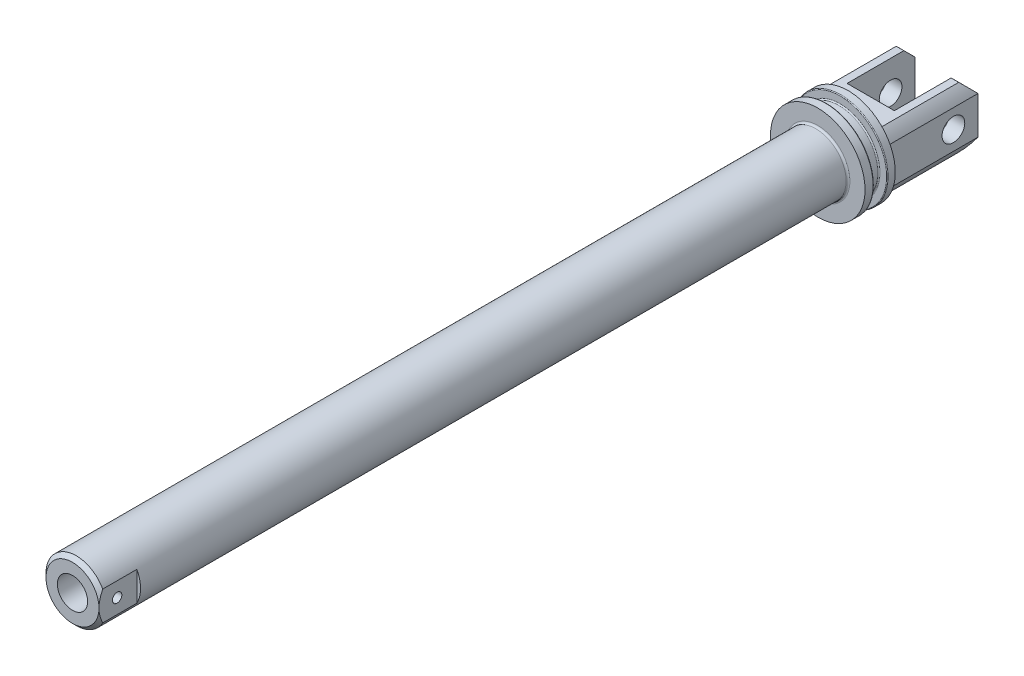
from build123d import *

# Parameters (mm, degrees)
SKETCH1_R               = 8
BOSS_EXTRUDE1_DEPTH     = 197
SKETCH2_R               = 12.5
BOSS_EXTRUDE2_DEPTH     = 8
SKETCH3_W               = 2.25
SKETCH3_H               = 3.6
SKETCH8_R               = 11.5
BOSS_EXTRUDE4_DEPTH     = 24
CUT_EXTRUDE1_DEPTH      = 198.791556948
CUT_EXTRUDE1_DEPTH_BACK = 198.791556948
SKETCH10_W              = 12.5
SKETCH10_H              = 21.605782088
CUT_EXTRUDE3_DEPTH      = 231.593256623
CUT_EXTRUDE3_DEPTH_BACK = 231.593256623
CUT_EXTRUDE5_START      = -24
CUT_EXTRUDE5_DEPTH      = 24
FILLET1_R               = 0.5
FILLET2_R               = 0.2
FILLET3_R               = 0.3
CHAMFER3_SIZE           = 1
CUT_EXTRUDE7_DEPTH      = 199.457804086
CUT_EXTRUDE7_DEPTH_BACK = 199.457804086
SKETCH15_W              = 2.199256875
SKETCH15_H              = 8
SKETCH15_W_2            = 2.880068719
SKETCH15_H_2            = 10
SKETCH14_R              = 3
CUT_EXTRUDE6_DEPTH      = 24
HOLE2_D                 = 8
HOLE2_DEPTH             = 7.5
M6_TAPPED_HOLE1_D       = 5
M6_TAPPED_HOLE1_DEPTH   = 18
M6_TAPPED_HOLE1_TIP     = 1.502151548
M3_TAPPED_HOLE1_D       = 2.5
M3_TAPPED_HOLE1_DEPTH   = 7.5
M3_TAPPED_HOLE1_TIP     = 0.751075774


with BuildPart() as part:
    # Sketch1 → Boss-Extrude1 (new body)
    with BuildSketch(Plane.XY):
        Circle(SKETCH1_R)
    extrude(amount=BOSS_EXTRUDE1_DEPTH)

    # Sketch2 → Boss-Extrude2 (add)
    with BuildSketch(Plane(origin=(0, 0, 0), x_dir=(-1, 0, 0), z_dir=(0, 0, -1))):
        Circle(SKETCH2_R)
    extrude(amount=BOSS_EXTRUDE2_DEPTH)

    # Sketch3 → Cut-Revolve1 (revolve, cut)
    with BuildSketch(Plane(origin=(0, 0, 0), x_dir=(1, 0, 0), z_dir=(0, 1, 0))):
        with Locations((-11.375, 4.1)):
            Rectangle(SKETCH3_W, SKETCH3_H)
    revolve(axis=Axis((0, 0, -10.00817261), (0, 0, 1)), mode=Mode.SUBTRACT)

    # Sketch8 → Boss-Extrude4 (add)
    with BuildSketch(Plane(origin=(0, 0, -8), x_dir=(-1, 0, 0), z_dir=(0, 0, -1))):
        Circle(SKETCH8_R)
    extrude(amount=BOSS_EXTRUDE4_DEPTH)

    # Sketch10 → Cut-Extrude1 (cut, two sides: drawn at the far end of the back side and taken through both)
    with BuildSketch(Plane(origin=(0, 0, 0), x_dir=(1, 0, 0), z_dir=(0, 1, 0)).offset(-CUT_EXTRUDE1_DEPTH_BACK)):
        with Locations((0, 24.802891044)):
            Rectangle(SKETCH10_W, SKETCH10_H)
    extrude(amount=CUT_EXTRUDE1_DEPTH + CUT_EXTRUDE1_DEPTH_BACK, mode=Mode.SUBTRACT)

    # Sketch11 → Cut-Extrude3 (cut, two sides: drawn at the far end of the back side and taken through both)
    with BuildSketch(Plane(origin=(0, -11.5, -32), x_dir=(0, 0, -1), z_dir=(-1, 0, 0)).offset(-CUT_EXTRUDE3_DEPTH_BACK)):
        Polygon((0.010981051, -16.5), (-3, -19.5), (-24, -19.5), (-24, -26.396557876), (1.498378991, -26.396557876), (1.498378991, -19.5), (0.010981051, -19.5), align=None)
        Polygon((-24, -3.5), (-24, 3.359688932), (2.769529036, 3.359688932), (2.769529036, -3.5), (1.498378991, -3.5), (0.010981051, -3.5), (0.010981051, -6.5), (-3, -3.5), align=None)
    extrude(amount=CUT_EXTRUDE3_DEPTH + CUT_EXTRUDE3_DEPTH_BACK, mode=Mode.SUBTRACT)

    # Sketch13 → Cut-Extrude5 (cut)
    with BuildSketch(Plane(origin=(0, 0, -32), x_dir=(-1, 0, 0), z_dir=(0, 0, -1)).offset(CUT_EXTRUDE5_START)):
        with BuildLine():
            Line((10.356157589, -5), (10.356157589, 5))
            ThreePointArc((10.356157589, 5), (11.5, 0), (10.356157589, -5))
        make_face()
        with BuildLine():
            Line((-10.356157589, -5), (-10.356157589, 5))
            ThreePointArc((-10.356157589, 5), (-11.5, 0), (-10.356157589, -5))
        make_face()
    extrude(amount=CUT_EXTRUDE5_DEPTH, mode=Mode.SUBTRACT)

    # Fillet1
    fillet1_edges = [part.edges().sort_by_distance(p)[0] for p in [
        (-8, 0, 0),
    ]]
    fillet(fillet1_edges, radius=FILLET1_R)

    # Fillet2
    fillet2_edges = [part.edges().sort_by_distance(p)[0] for p in [
        (12.5, 0, -2.3),
        (12.5, 0, -5.9),
    ]]
    fillet(fillet2_edges, radius=FILLET2_R)

    # Fillet3
    fillet3_edges = [part.edges().sort_by_distance(p)[0] for p in [
        (10.25, 0, -2.3),
        (10.25, 0, -5.9),
    ]]
    fillet(fillet3_edges, radius=FILLET3_R)

    # Chamfer3
    chamfer3_edges = [part.edges().sort_by_distance(p)[0] for p in [
        (-8, 0, 197),
    ]]
    chamfer(chamfer3_edges, length=CHAMFER3_SIZE)

    # Sketch15 → Cut-Extrude7 (cut, two sides: drawn at the far end of the back side and taken through both)
    with BuildSketch(Plane(origin=(0, 8, 0), x_dir=(1, 0, 0), z_dir=(0, 1, 0)).offset(-CUT_EXTRUDE7_DEPTH_BACK)):
        with Locations((-8.099628438, -191)):
            Rectangle(SKETCH15_W, SKETCH15_H)
        with BuildLine():
            Line((-8.5, -153.05), (-9.470215056, -153.05))
            Line((-9.470215056, -153.05), (-9.470215056, -177.95))
            Line((-9.470215056, -177.95), (-8.5, -177.95))
            ThreePointArc((-8.5, -177.95), (-6.732233047, -177.217766953), (-6, -175.45))
            Line((-6, -175.45), (-6, -155.55))
            ThreePointArc((-6, -155.55), (-6.732233047, -153.782233047), (-8.5, -153.05))
        make_face()
        with Locations((8.44003436, -192)):
            Rectangle(SKETCH15_W_2, SKETCH15_H_2)
    extrude(amount=CUT_EXTRUDE7_DEPTH + CUT_EXTRUDE7_DEPTH_BACK, mode=Mode.SUBTRACT)

    # Sketch14 → Cut-Extrude6 (cut)
    with BuildSketch(Plane(origin=(10.356157589, 0, 0), x_dir=(0, 0, -1), z_dir=(1, 0, 0))):
        with Locations(Location((25.5, 0, 0), (0, 0, 90))):
            Circle(SKETCH14_R)
    extrude(amount=-CUT_EXTRUDE6_DEPTH, mode=Mode.SUBTRACT)

    # Hole2
    with Locations(Plane.XY.offset(197)):
        with Locations((0, 0)):
            Hole(HOLE2_D / 2, depth=HOLE2_DEPTH)

    # M6 Tapped Hole1
    with Locations(Plane.XY.offset(197)):
        with Locations((0, 0)):
            Hole(M6_TAPPED_HOLE1_D / 2, depth=M6_TAPPED_HOLE1_DEPTH)
            with Locations((0, 0, -(M6_TAPPED_HOLE1_DEPTH + M6_TAPPED_HOLE1_TIP / 2))):  # 118° drill point
                Cone(0, M6_TAPPED_HOLE1_D / 2, M6_TAPPED_HOLE1_TIP, mode=Mode.SUBTRACT)

    # M3 Tapped Hole1
    with Locations(Plane(origin=(7, 0, 0), x_dir=(0, 0, -1), z_dir=(1, 0, 0))):
        with Locations((-192.2, 0)):
            Hole(M3_TAPPED_HOLE1_D / 2, depth=M3_TAPPED_HOLE1_DEPTH)
            with Locations((0, 0, -(M3_TAPPED_HOLE1_DEPTH + M3_TAPPED_HOLE1_TIP / 2))):  # 118° drill point
                Cone(0, M3_TAPPED_HOLE1_D / 2, M3_TAPPED_HOLE1_TIP, mode=Mode.SUBTRACT)


solid = part.part
